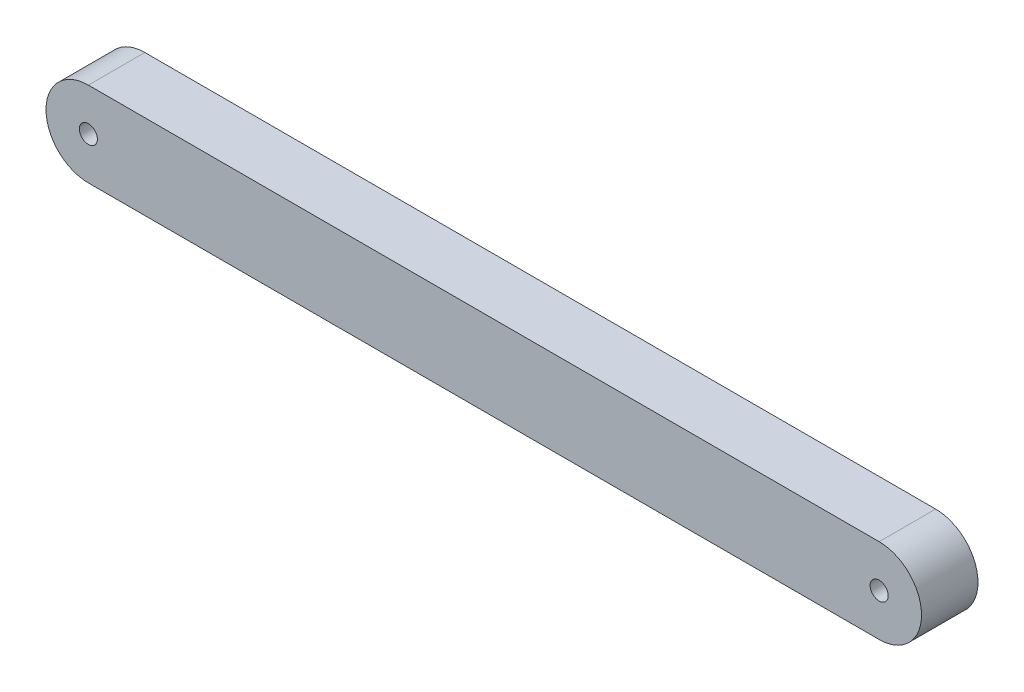
SolidWorks part; units mm, degrees
ref_plane "前视基准面" through (0, 0, 0) normal (0, 0, 1) x (1, 0, 0)
ref_plane "上视基准面" through (0, 0, 0) normal (0, 1, 0) x (1, 0, 0)
ref_plane "右视基准面" through (0, 0, 0) normal (1, 0, 0) x (0, 0, -1)
other "Configuration Table"
sketch "草图1" plane through (0, 0, 0) normal (0, 0, 1) x (1, 0, 0)
  line L0 (-140, 15) -> (140, 15)
  line L1 (140, -15) -> (-140, -15)
  arc A0 (140, 15) -> (140, -15) centre (140, 0) cw
  arc A1 (-140, -15) -> (-140, 15) centre (-140, 0) cw
  point P0 (0, 0)
  dimension "D1" = 15
  dimension "D2" = 140
  dimension "D3" = 280
extrude "凸台-拉伸1" add sketch "草图1" against normal mid plane 20
sketch "草图2" plane through (0, 0, 0) normal (0, 0, 1) x (1, 0, 0)
  circle A0 centre (-140, 0) radius 3.2
  circle A1 centre (140, 0) radius 3.2
  point P0 (0, 0)
  dimension "D1" = 6.4
  dimension "D2" = 6.4
  dimension "D3" = 140
  dimension "D4" = 280
extrude "切除-拉伸1" cut sketch "草图2" against normal mid plane 50
